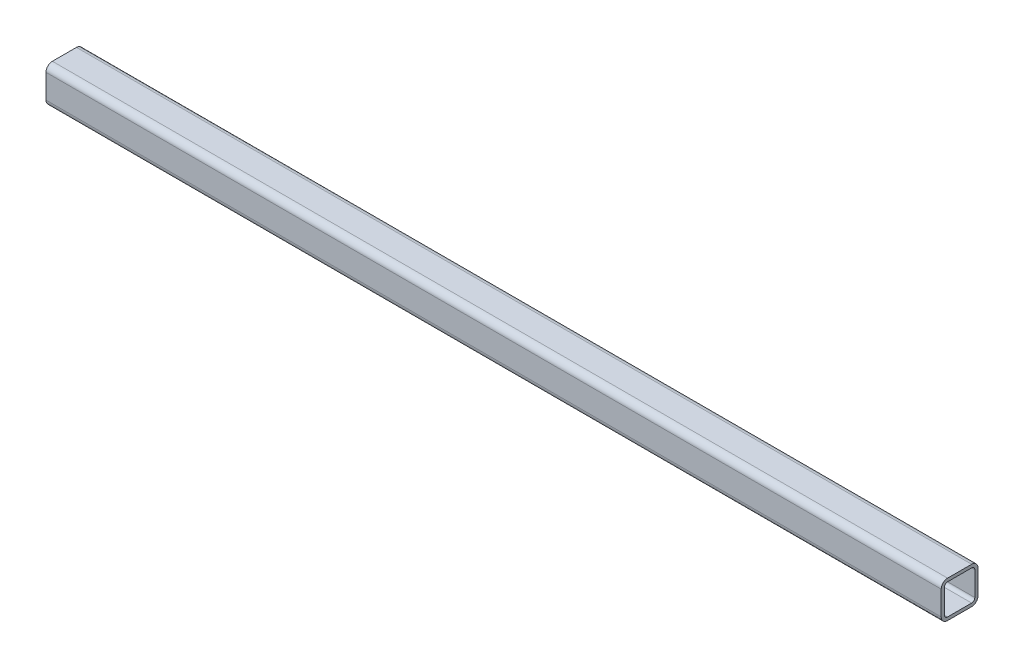
from build123d import *

# Parameters (mm, degrees)
MEMBER_1_DEPTH = 730


with BuildPart() as part:
    # Sketch1 → Member 1 (new body)
    with BuildSketch(Plane(origin=(0, 0, 0), x_dir=(0, 0, -1), z_dir=(1, 0, 0))):
        with BuildLine():
            Line((-9.8, -15), (9.8, -15))
            ThreePointArc((9.8, -15), (13.476955262, -13.476955262), (15, -9.8))
            Line((15, -9.8), (15, 9.8))
            ThreePointArc((15, 9.8), (13.476955262, 13.476955262), (9.8, 15))
            Line((9.8, 15), (-9.8, 15))
            ThreePointArc((-9.8, 15), (-13.476955262, 13.476955262), (-15, 9.8))
            Line((-15, 9.8), (-15, -9.8))
            ThreePointArc((-15, -9.8), (-13.476955262, -13.476955262), (-9.8, -15))
        make_face()
        with BuildLine():
            Line((-9.8, -12.4), (9.8, -12.4))
            ThreePointArc((9.8, -12.4), (11.638477631, -11.638477631), (12.4, -9.8))
            Line((12.4, -9.8), (12.4, 9.8))
            ThreePointArc((12.4, 9.8), (11.638477631, 11.638477631), (9.8, 12.4))
            Line((9.8, 12.4), (-9.8, 12.4))
            ThreePointArc((-9.8, 12.4), (-11.638477631, 11.638477631), (-12.4, 9.8))
            Line((-12.4, 9.8), (-12.4, -9.8))
            ThreePointArc((-12.4, -9.8), (-11.638477631, -11.638477631), (-9.8, -12.4))
        make_face(mode=Mode.SUBTRACT)
    extrude(amount=MEMBER_1_DEPTH)


solid = part.part
